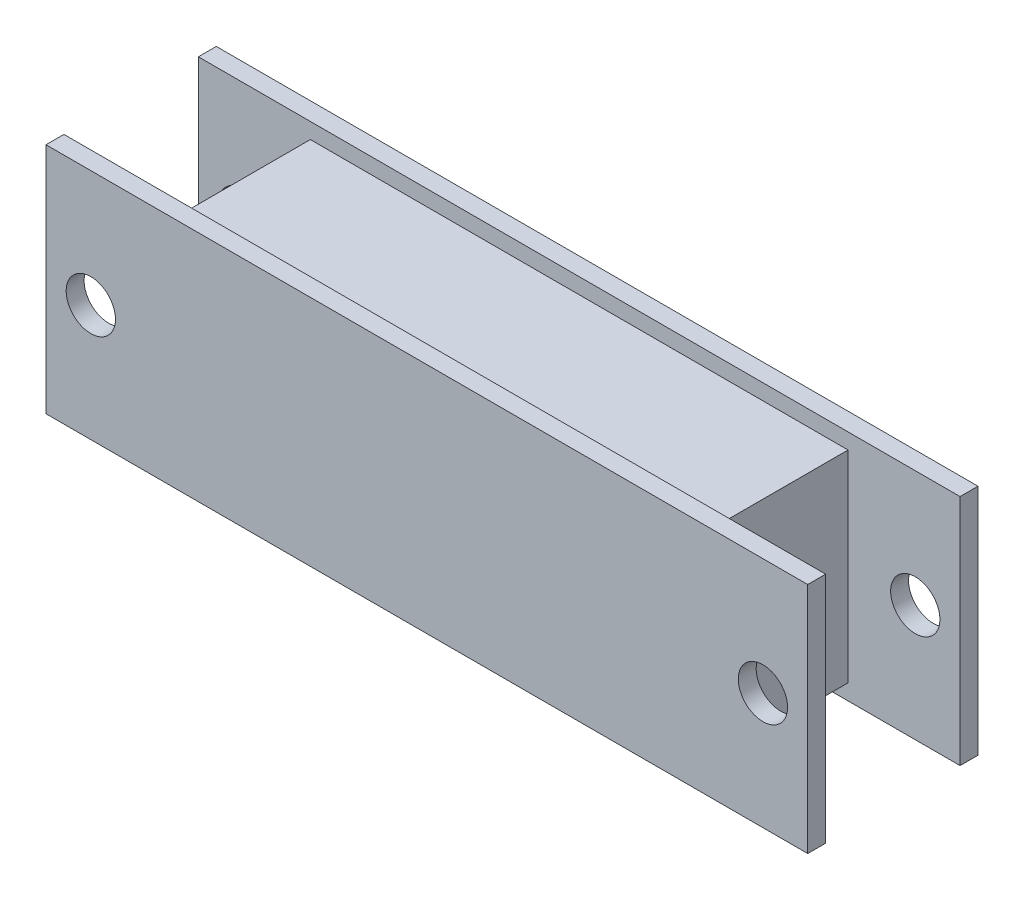
from build123d import *

# Parameters (mm, degrees)
SKETCH_1_W          = 120
SKETCH_1_H          = 45
EXTRUDE_1_DEPTH     = 15
SKETCH_2_W          = 170
SKETCH_2_H          = 52
EXTRUDE_2_DEPTH     = 4
SKETCH_3_R          = 5.5
CUT_EXTRUDE_1_DEPTH = 97.669540187


with BuildPart() as part:
    # 草图1 → 凸台-拉伸1 (new, symmetric)
    with BuildSketch(Plane.XY):
        Rectangle(SKETCH_1_W, SKETCH_1_H)
    extrude(amount=EXTRUDE_1_DEPTH, both=True)

    # 草图2 → 凸台-拉伸2 (add)
    with BuildSketch(Plane.XY.offset(15)):
        Rectangle(SKETCH_2_W, SKETCH_2_H)
    extrude_2 = extrude(amount=EXTRUDE_2_DEPTH)

    # 镜向1: 凸台-拉伸2 across plane
    add(extrude_2.mirror(Plane.XY))

    # 草图3 → 切除-拉伸1 (cut, through all)
    with BuildSketch(Plane.XY.offset(19)):
        with Locations((-75, 0)):
            Circle(SKETCH_3_R)
        with Locations(Location((75, 0, 0), (0, 0, 180))):
            Circle(SKETCH_3_R)
    extrude(amount=-CUT_EXTRUDE_1_DEPTH, mode=Mode.SUBTRACT)


solid = part.part
